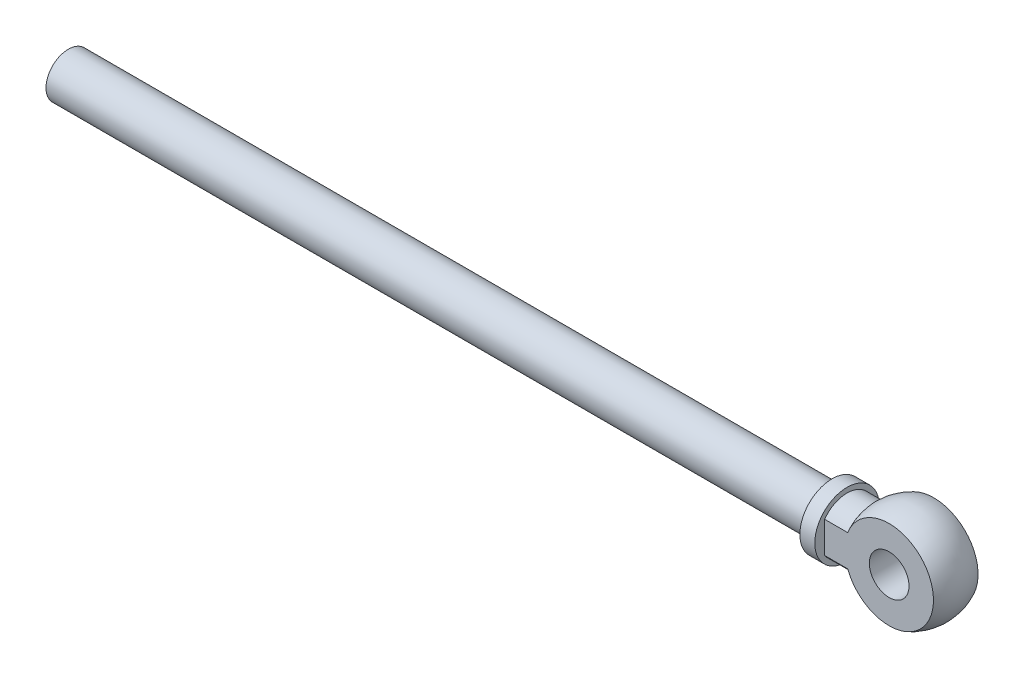
from build123d import *

# Parameters (mm, degrees)
SKETCH_2_W          = 36.907420495
SKETCH_2_H          = 136.774558304
CUT_EXTRUDE_1_DEPTH = 789.178279325
SKETCH_3_R          = 20
CUT_EXTRUDE_2_DEPTH = 754.674332852


with BuildPart() as part:
    # Sketch 1 → Revolve 1 (revolve)
    with BuildSketch(Plane.XY, mode=Mode.PRIVATE) as revolve_1_sk:
        with BuildLine():
            Line((-750, 0), (-750, 22.5))
            Line((-750, 22.5), (20, 22.5))
            Line((20, 22.5), (20, 32.5))
            Line((20, 32.5), (35, 32.5))
            Line((35, 32.5), (35, 27.5))
            Line((35, 27.5), (58.241767279, 27.5))
            ThreePointArc((58.241767279, 27.5), (114.354239164, 47.895258826), (150, 0))
            Line((150, 0), (-750, 0))
        make_face()
    revolve(revolve_1_sk.sketch.rotate(Axis((-750, 0, 0), (1, 0, 0)), 90), axis=Axis((-750, 0, 0), (1, 0, 0)))

    # Sketch 2 → Cut-Extrude 1 (cut, through all)
    with BuildSketch(Plane(origin=(35, 0, 0), x_dir=(0, 0, -1), z_dir=(1, 0, 0))):
        with Locations((40.953710247, 0)):
            Rectangle(SKETCH_2_W, SKETCH_2_H)
        with Locations((-40.953710247, 0)):
            Rectangle(SKETCH_2_W, SKETCH_2_H)
    extrude(amount=CUT_EXTRUDE_1_DEPTH, mode=Mode.SUBTRACT)

    # Sketch 3 → Cut-Extrude 2 (cut, through all)
    with BuildSketch(Plane(origin=(0, 0, -22.5), x_dir=(-1, 0, 0), z_dir=(0, 0, -1))):
        with Locations((-100, 0)):
            Circle(SKETCH_3_R)
    extrude(amount=-CUT_EXTRUDE_2_DEPTH, mode=Mode.SUBTRACT)


solid = part.part
